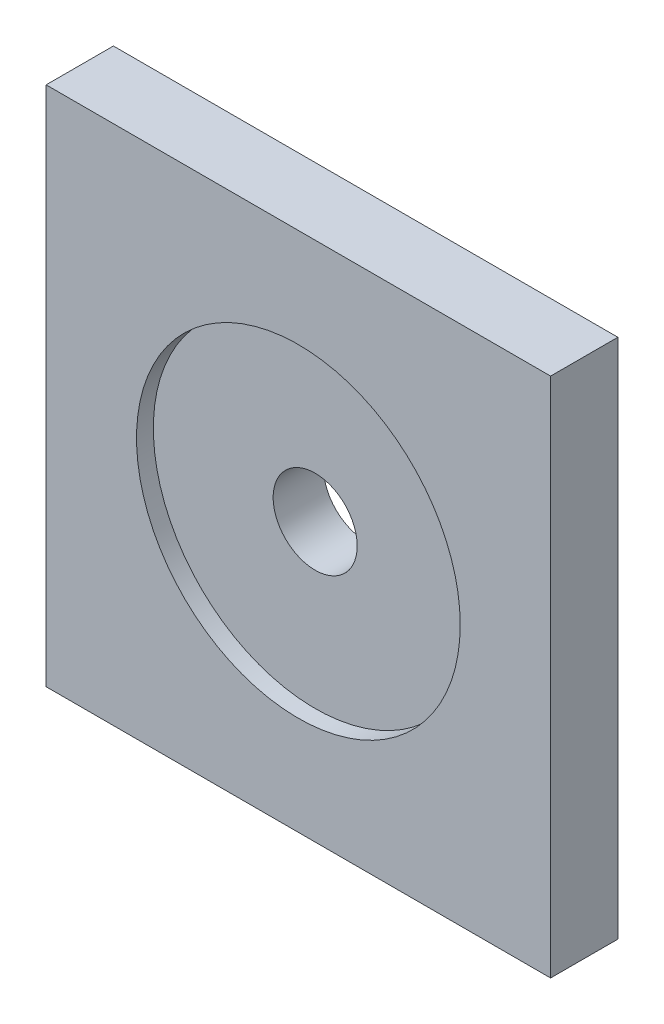
SolidWorks part; units mm, degrees
ref_plane "Front Plane" through (0, 0, 0) normal (0, 0, 1) x (1, 0, 0)
ref_plane "Top Plane" through (0, 0, 0) normal (0, 1, 0) x (1, 0, 0)
ref_plane "Right Plane" through (0, 0, 0) normal (1, 0, 0) x (0, 0, -1)
sketch "Sketch1" plane through (0, 0, 0) normal (0, 0, 1) x (1, 0, 0)
  line L1 (-30, 31) -> (30, 31)
  line L2 (-30, 31) -> (-30, -31)
  line L3 (-30, -31) -> (30, -31)
  line L4 (30, 31) -> (30, -31)
  line L5 (-30, 31) -> (30, -31) construction
  line L6 (-30, -31) -> (30, 31) construction
  point P0 (0, 0)
  dimension "D1" = 60
  dimension "D2" = 62
extrude "Boss-Extrude1" add sketch "Sketch1" along normal blind 8
sketch "Sketch2" plane through (0, 0, 8) normal (0, 0, 1) x (1, 0, 0)
  line L0 (0, -31.1624) -> (0, -11.1624) construction
  line L1 (-5, -31.1624) -> (-5, -11.1624)
  line L2 (5, -31.1624) -> (5, -11.1624)
  line L4 (30, 31) -> (-30, 31) construction
  arc A1 (-5, -31.1624) -> (5, -31.1624) centre (0, -31.1624) ccw
  arc A2 (5, -11.1624) -> (-5, -11.1624) centre (0, -11.1624) ccw
  point P2 (0, -21.1624)
  point P13 (0, 31)
  dimension "D1" = 20
  dimension "D2" = 10
sketch "Sketch3" plane through (0, 0, 8) normal (0, 0, 1) x (1, 0, 0)
  circle A0 centre (0, 0) radius 19.25
  dimension "D1" = 38.5
extrude "Cut-Extrude1" cut sketch "Sketch3" against normal blind 2
sketch "Sketch4" plane through (0, 0, 6) normal (0, 0, 1) x (1, 0, 0)
  circle A0 centre (0, 0) radius 5
  dimension "D1" = 10
extrude "Cut-Extrude2" cut sketch "Sketch4" against normal through all
